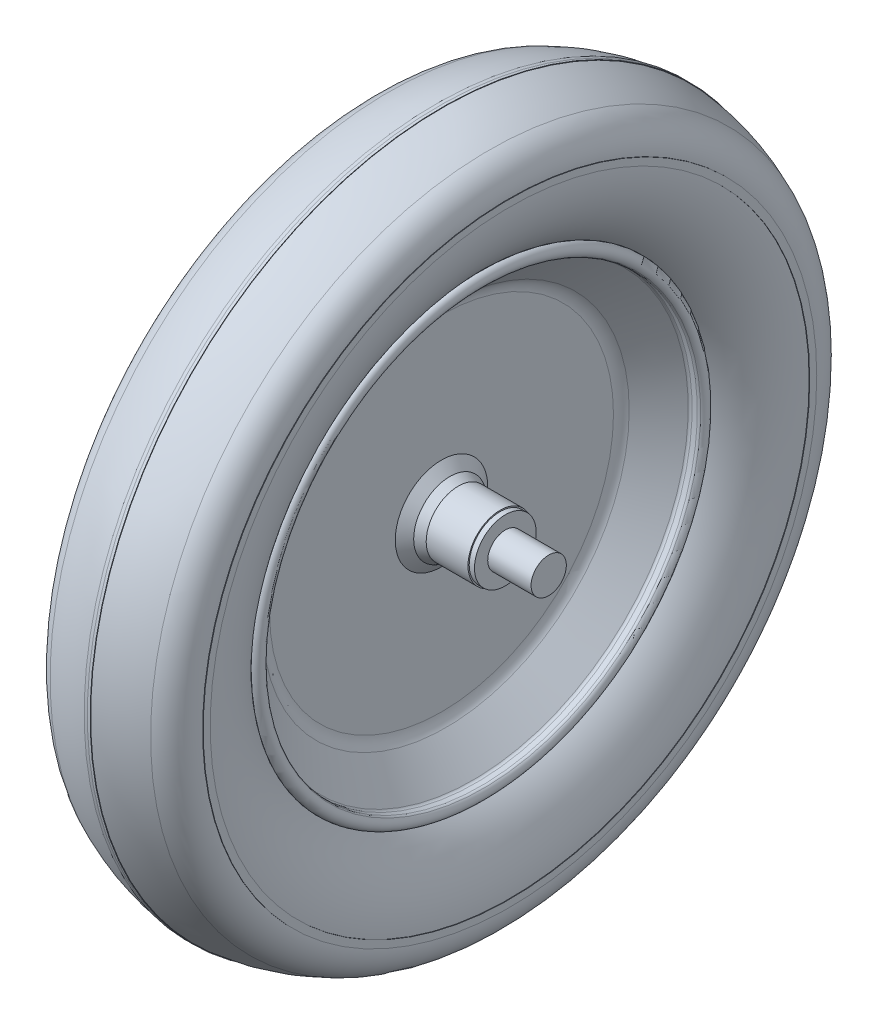
from build123d import *

# Parameters (mm, degrees)
BOSS_EXTRUDE1_DEPTH      = 25
BOSS_EXTRUDE1_DEPTH_BACK = 100
SKETCH3_R                = 10


with BuildPart() as part:
    # Sketch1 → Revolve1 (revolve)
    with BuildSketch(Plane.XY, mode=Mode.PRIVATE) as revolve1_sk:
        with BuildLine():
            Line((41.387744688, -19.739643253), (42.887744688, -19.739643253))
            Line((42.887744688, -19.739643253), (42.887744688, -12.239643253))
            Line((42.887744688, -12.239643253), (39.887744688, -12.239643253))
            Line((39.887744688, -12.239643253), (39.887744688, -11.539643253))
            Line((39.887744688, -11.539643253), (16.187744688, -11.539643253))
            Line((16.187744688, -11.539643253), (11.387744688, -9.239643253))
            Line((11.387744688, -9.239643253), (6.687744688, -3.489643253))
            Line((6.687744688, -3.489643253), (6.687744688, 67.794317568))
            ThreePointArc((6.687744688, 67.794317568), (7.31132558, 71.270344714), (9.104297631, 74.312855038))
            Line((9.104297631, 74.312855038), (24.577677456, 92.314064241))
            ThreePointArc((24.577677456, 92.314064241), (25.259925434, 92.827967127), (26.094366868, 93.010356747))
            Line((26.094366868, 93.010356747), (29.048594764, 93.010356747))
            ThreePointArc((29.048594764, 93.010356747), (29.773764695, 93.146455308), (30.400240041, 93.536228175))
            ThreePointArc((30.400240041, 93.536228175), (31.552866637, 97.414843022), (28.676192717, 100.260356747))
            Line((28.676192717, 100.260356747), (28.473245406, 98.760356747))
            ThreePointArc((28.473245406, 98.760356747), (30.118425574, 96.964644724), (29.386506083, 94.641824604))
            ThreePointArc((29.386506083, 94.641824604), (29.229887247, 94.544381387), (29.048594764, 94.510356747))
            Line((29.048594764, 94.510356747), (26.094366868, 94.510356747))
            ThreePointArc((26.094366868, 94.510356747), (24.634094359, 94.191174912), (23.440160398, 93.291844861))
            Line((23.440160398, 93.291844861), (7.604297631, 74.868935207))
            ThreePointArc((7.604297631, 74.868935207), (5.81132558, 71.826424883), (5.187744688, 68.350397737))
            Line((5.187744688, 68.350397737), (5.187744688, -4.024687802))
            Line((5.187744688, -4.024687802), (10.437993534, -10.447864582))
            Line((10.437993534, -10.447864582), (15.846922936, -13.039643253))
            Line((15.846922936, -13.039643253), (38.387744688, -13.039643253))
            Line((38.387744688, -13.039643253), (38.387744688, -13.739643253))
            Line((38.387744688, -13.739643253), (38.387744688, -19.739643253))
            Line((38.387744688, -19.739643253), (41.387744688, -19.739643253))
        make_face()
    revolve(revolve1_sk.sketch.rotate(Axis((-118.954757241, -29.739643253, 0), (1, 0, 0)), 90), axis=Axis((-118.954757241, -29.739643253, 0), (1, 0, 0)))


with BuildPart() as body_2:
    # Sketch2 → Revolve2 (revolve)
    with BuildSketch(Plane.XY, mode=Mode.PRIVATE) as revolve2_sk:
        with BuildLine():
            Line((28.597859248, 100.291346958), (28.394911937, 98.791346958))
            Line((28.394911937, 98.791346958), (28.394911937, 95.313479471))
            ThreePointArc((28.394911937, 95.313479471), (28.248465327, 94.959926081), (27.894911937, 94.813479471))
            Line((27.894911937, 94.813479471), (27.735671368, 94.813479471))
            ThreePointArc((27.735671368, 94.813479471), (26.321457806, 95.399265909), (25.735671368, 96.813479471))
            Line((25.735671368, 96.813479471), (25.735671368, 100.854321086))
            ThreePointArc((25.735671368, 100.854321086), (25.902079477, 101.653033035), (26.373612145, 102.318832838))
            ThreePointArc((26.373612145, 102.318832838), (38.305289981, 119.366106553), (42.209606894, 139.804569961))
            Line((42.209606894, 139.804569961), (42.22028084, 145.141002184))
            ThreePointArc((42.22028084, 145.141002184), (39.585207528, 153.827911455), (32.522271283, 159.530624463))
            ThreePointArc((32.522271283, 159.530624463), (18.333714714, 164.452669108), (3.497859248, 166.784846971))
            Line((3.497859248, 166.784846971), (3.497859248, 169.791346958))
            ThreePointArc((3.497859248, 169.791346958), (18.933986878, 167.39482088), (33.697859248, 162.291346958))
            ThreePointArc((33.697859248, 162.291346958), (42.320828696, 155.126855217), (45.197859248, 144.291346958))
            Line((45.197859248, 144.291346958), (45.497859248, 144.291346958))
            Line((45.497859248, 144.291346958), (45.497859248, 140.291346958))
            Line((45.497859248, 140.291346958), (45.197859248, 140.291346958))
            ThreePointArc((45.197859248, 140.291346958), (41.197859248, 118.506846958), (28.597859248, 100.291346958))
        make_face()
    revolve(revolve2_sk.sketch.rotate(Axis((51.301478022, -29.739643253, 0), (-1, 0, 0)), 90), axis=Axis((51.301478022, -29.739643253, 0), (-1, 0, 0)))


with BuildPart() as body_3:
    # Mirror8: mirrored copy
    add(part.part.mirror(Plane(origin=(5.187744688, -4.024687802, 0), x_dir=(0, 0, 1), z_dir=(1, 0, 0))))


with BuildPart() as body_4:
    # Mirror8 2: mirrored copy
    add(body_2.part.mirror(Plane(origin=(5.187744688, -4.024687802, 0), x_dir=(0, 0, 1), z_dir=(1, 0, 0))))


with BuildPart() as part_1:
    add(part.part)

    add(body_3.part)  # Boss-Extrude1 merges body 3

    add(body_2.part)  # Boss-Extrude1 merges body 2

    add(body_4.part)  # Boss-Extrude1 merges body 4
    # Sketch3 → Boss-Extrude1 (add, two sides: drawn at the far end of the back side and taken through both)
    with BuildSketch(Plane.ZY.offset(32.512255312).offset(-BOSS_EXTRUDE1_DEPTH_BACK)):
        with Locations((0, -29.739643253)):
            Circle(SKETCH3_R)
    extrude(amount=BOSS_EXTRUDE1_DEPTH + BOSS_EXTRUDE1_DEPTH_BACK)


solid = part_1.part
